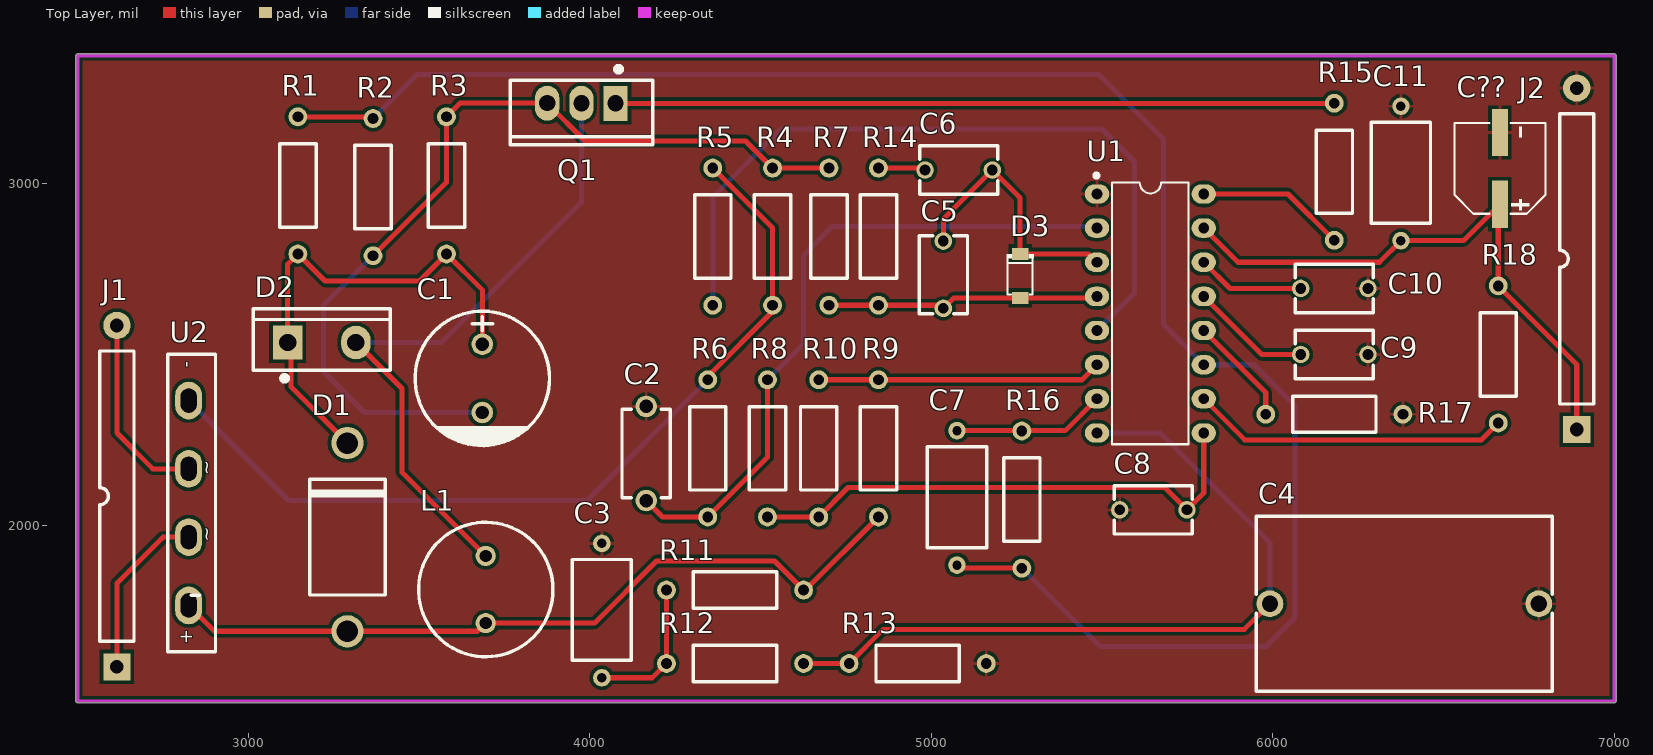
[diagram p0: Top Layer view]
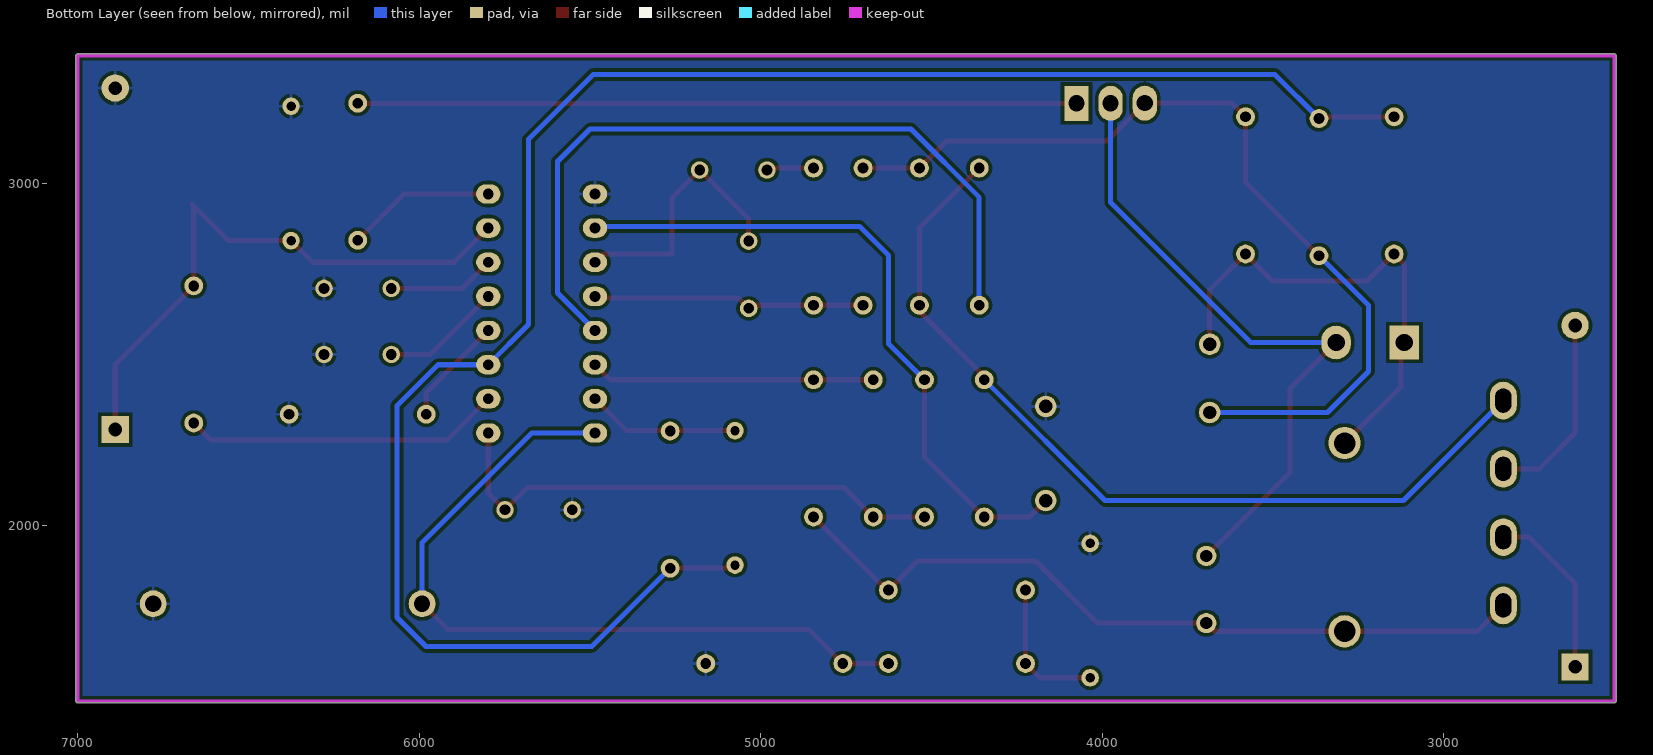
[diagram p1: Bottom Layer view, seen from below]
# Altium PCB MISC82375-2.PcbDoc
Units mil, origin at the board's own origin, x right, y up, seen from the top; angles counter-clockwise.
Board outline 4510.03 x 1900.03 mil, 2 copper layers (Top Layer, Bottom Layer); 39 components, 26 nets, 95 pads, 0 vias.

## Layer stack, top to bottom (the 12.6 mil dielectric is the usual default, probably not edited)
Top Solder: solder mask 0.4, Solder Resist, Dk 3.5
Top Layer: signal copper 1.4
Dielectric 1: dielectric 12.6, FR-4, Dk 4.8
Bottom Layer: signal copper 1.4
Bottom Solder: solder mask 0.4, Solder Resist, Dk 3.5

## Board outline
2494.99,1485 ccw(c2500,1485) 2500,1479.98 7000,1479.98 ccw(c7000,1485) 7005.02,1485 7005.02,3375 ccw(c7000,3375) 7000,3380.01 2500,3380.01 ccw(c2500,3375) 2494.99,3375

## Design rules (kind name [scope] priority, off if disabled: settings)
Clearance [All] p1: gap=10
MinimumSolderMaskSliver [All] p1: minsoldermaskwidth=0
PolygonConnect [All] p1: connectstyle=Relief reliefconductorwidth=10 reliefentries=4 polygonreliefangle="90 Angle" airgapwidth=10
RoutingVias [All] p1: holewidth=28 width=50 viastyle="Through Hole" minholewidth=28 minwidth=50 maxholewidth=28 maxwidth=50
SilkToSilkClearance [All] p1: silktosilkclearance=0
SilkToSolderMaskClearance [IsPad] p1: minsilkscreentomaskgap=0 clearancetoexposedcopper=TRUE
SolderMaskExpansion [All] p1: expansion=4
Width [All] p1: maxlimit=30 minlimit=10 preferedwidth=10
27 further rules are at their usual default settings.

## Components (designator, comment, footprint, x,y, rotation, side; value= is the part's Value field where it differs from the comment)
C1 "LKME1402A101MF" CAP-TH_BD10.0-P5.00-D1.0-FD 3685,2430 r270 top
C2 "KJKF222M2FF7035A075E" CAP-TH_L6.5-W3.5-P7.50-D1.0 4165,2210 r270 top
C3 "KY1102M400VAC70Y10093" CAP-TH_L7.5-W4.5-P10.00-D0.6 4035,1750 r270 top
C4 "CBB21-400V/255JP20" CAP-TH_L22.0-W12.5-P20.00-D0.7-FD 6385,1770 r180 top
C5 "178MU0002" CAP-TH_L5.8-W3.6-P5.0-D0.6 5035,2733.42 r90 top
C6 "178MU0002" CAP-TH_L5.8-W3.6-P5.0-D0.6 5080,3040 r180 top
C7 "KY1102M400VAC70Y10093" CAP-TH_L7.5-W4.5-P10.00-D0.6 5075,2080 r270 top
C8 "178MU0002" CAP-TH_L5.8-W3.6-P5.0-D0.6 5650,2045 r0 top
C9 "178MU0002" CAP-TH_L5.8-W3.6-P5.0-D0.6 6180,2500 r0 top
C10 "178MU0002" CAP-TH_L5.8-W3.6-P5.0-D0.6 6180,2693.43 r0 top
C11 "KY1102M400VAC70Y10093" CAP-TH_L7.5-W4.5-P10.00-D0.6 6375,3030 r270 top
C?? "RVE100UF35V67RV0072" CAP-SMD_BD6.3-L6.6-W6.6-LS7.6-FD-1 6665,3044.89 r90 top
D1 "1N5406_C5338388" DO-27_BD5.2-L8.9-P12.90-D1.5-RD 3290,1965 r270 top
D2 "GC3D10060A" TO-220-2_L10.2-W4.5-P5.08-L-A 3215,2535 r0 top
D3 "BZT52C8V2_C19077406" SOD-123_L2.7-W1.6-LS3.7-RD 5260,2730 r270 top
J1 "HOLE" DIP2 2615,1585 r90 top
J2 "HOLE" DIP2 6890,2280 r90 top
L1 "XR8*10-101K-L" IND-TH_BD10.0-P5.00-D0.6 3695,1811.57 r90 top
Q1 "IRF530NPBF" TO-220-3_L10.0-W4.5-P2.54-L 3975.01,3235.61 r180 top
R1 "MF1/4W-100K±1%-OT26" RES-TH_BD2.7-L6.2-P10.20-D0.4 3145,2995 r270 top
R2 "MF1/4W-100K±1%-OT26" RES-TH_BD2.7-L6.2-P10.20-D0.4 3365,2990 r90 top
R3 "MF1/4W-100K±1%-OT26" RES-TH_BD2.7-L6.2-P10.20-D0.4 3580,2995 r270 top
R4 "MF1/4W-100K±1%-OT26" RES-TH_BD2.7-L6.2-P10.20-D0.4 4535,2845 r90 top
R5 "MF1/4W-100K±1%-OT26" RES-TH_BD2.7-L6.2-P10.20-D0.4 4360,2845 r90 top
R6 "MF1/4W-100K±1%-OT26" RES-TH_BD2.7-L6.2-P10.20-D0.4 4345,2225 r90 top
R7 "MF1/4W-100K±1%-OT26" RES-TH_BD2.7-L6.2-P10.20-D0.4 4700,2845 r90 top
R8 "MF1/4W-100K±1%-OT26" RES-TH_BD2.7-L6.2-P10.20-D0.4 4520,2225 r90 top
R9 "MF1/4W-100K±1%-OT26" RES-TH_BD2.7-L6.2-P10.20-D0.4 4845,2225 r270 top
R10 "MF1/4W-100K±1%-OT26" RES-TH_BD2.7-L6.2-P10.20-D0.4 4670,2225 r270 top
R11 "MF1/4W-100K±1%-OT26" RES-TH_BD2.7-L6.2-P10.20-D0.4 4425,1810 r0 top
R12 "MF1/4W-100K±1%-OT26" RES-TH_BD2.7-L6.2-P10.20-D0.4 4425,1595 r0 top
R13 "MF1/4W-100K±1%-OT26" RES-TH_BD2.7-L6.2-P10.20-D0.4 4960,1595 r180 top
R14 "MF1/4W-100K±1%-OT26" RES-TH_BD2.7-L6.2-P10.20-D0.4 4845,2845 r90 top
R15 "MF1/4W-100K±1%-OT26" RES-TH_BD2.7-L6.2-P10.20-D0.4 6180,3035 r270 top
R16 "MF1/4W-100K±1%-OT26" RES-TH_BD2.7-L6.2-P10.20-D0.4 5265,2075 r270 top
R17 "MF1/4W-100K±1%-OT26" RES-TH_BD2.7-L6.2-P10.20-D0.4 6180,2325 r0 top
R18 "MF1/4W-100K±1%-OT26" RES-TH_BD2.7-L6.2-P10.20-D0.4 6660,2500 r90 top
U1 "UC3854N" PDIP-16_L19.3-W6.4-P2.54-LS7.94-BL 5641.3,2620 r270 top
U2 "GBU8K" GBU_4P-L22.0-W3.5-P5.08-GBU4K 2825,2065 r270 top

## Footprints (in the part's own frame and the unit in brackets; to place one, negate y for a bottom-side part, rotate by r counter-clockwise, add the part's x,y. Pads: shape width x height; smd on the part's side, far side on the other; paste and mask are expansions set on the pad)
CAP-SMD_BD6.3-L6.6-W6.6-LS7.6-FD-1 [mm]
  rect 3.5x1.2 smd: 1(-2.67,0) 2(2.67,0)
  silkscreen extent -3.38,-3.38 3.38,3.38
CAP-TH_BD10.0-P5.00-D1.0-FD [mm]
  round 1.6 hole 1: 1(-2.54,0) 2(2.54,0)
  silkscreen extent -5,-5 5.08,5
CAP-TH_L5.8-W3.6-P5.0-D0.6 [mm]
  round 1.3 hole 0.8 paste+0 mask+0.05: 1(-2.5,0)
  round 1.3 hole 0.8 copper offset 0,0 paste+0 mask+0.05: 2(2.5,0)
  silkscreen extent -2.9,-1.8 2.9,1.8
CAP-TH_L6.5-W3.5-P7.50-D1.0 [mm]
  round 1.6 hole 1: 1(-3.5,0) 2(3.5,0)
  silkscreen extent -3.3,-1.8 3.3,1.8
CAP-TH_L7.5-W4.5-P10.00-D0.6 [mm]
  round 1.3 hole 0.7: 1(-5,0) 2(5,0)
  silkscreen extent -3.8,-2.2 3.7,2.2
CAP-TH_L22.0-W12.5-P20.00-D0.7-FD [mm]
  round 2 hole 1.2: 1(-10,0) 2(10,0)
  silkscreen extent -11,-6.5 11,6.5
DIP2 [mil]
  rect 80x80 hole 40: 1(0,0)
  round 80 hole 40: 2(1000,0)
  silkscreen extent 75,-50 925,50
DO-27_BD5.2-L8.9-P12.90-D1.5-RD [mm]
  round 2.4 hole 1.6: 1(-7,0) 2(7,0)
  silkscreen extent -4.3,-2.8 4.3,2.8
GBU_4P-L22.0-W3.5-P5.08-GBU4K [mm]
  oval 2.8x2 hole 1.2 slot 1.8 at 0 deg: 1(-7.62,0) 2(-2.54,0) 3(2.54,0) 4(7.62,0)
  silkscreen extent -11.05,-1.56 11.05,2
IND-TH_BD10.0-P5.00-D0.6 [mm]
  round 1.5 hole 0.9 paste+0 mask+0.05: 1(-2.5,0) 2(2.5,0)
  silkscreen extent -5,-5 5,5
PDIP-16_L19.3-W6.4-P2.54-LS7.94-BL [mm]
  oval 1.44x1.8 hole 0.8: 1(-8.89,-3.97) 2(-6.35,-3.97) 3(-3.81,-3.97) 4(-1.27,-3.97) 5(1.27,-3.97) 6(3.81,-3.97) 7(6.35,-3.97) 8(8.89,-3.97) 9(8.89,3.97) 10(6.35,3.97) 11(3.81,3.97) 12(1.27,3.97) 13(-1.27,3.97) 14(-3.81,3.97) 15(-6.35,3.97) 16(-8.89,3.97)
  silkscreen extent -10.41,-4.17 9.73,2.84
RES-TH_BD2.7-L6.2-P10.20-D0.4 [mm]
  round 1.4 hole 0.8 copper offset 0,0: 1(-5.1,0) 2(5.1,0)
  silkscreen extent -3.1,-1.35 3.1,1.35
SOD-123_L2.7-W1.6-LS3.7-RD [mm]
  rect 0.91x1.22 smd: 1(-1.635,0) 2(1.635,0)
  silkscreen extent -1.6,-1 1.38,1
TO-220-2_L10.2-W4.5-P5.08-L-A [mm]
  rect 2.2x2.5 hole 1.3: 1(-2.54,0)
  oval 2.2x2.5 hole 1.3: 3(2.54,0)
  silkscreen extent -5.1,-2.86 5.1,2.5
TO-220-3_L10.0-W4.5-P2.54-L [mm]
  rect 1.8x2.6 hole 1.2: 1(-2.54,0.005)
  oval 1.8x2.6 hole 1.2: 2(0,0.005)
  oval 1.8x2.6 hole 1.2 copper offset 0,0: 3(2.54,-0.005)
  silkscreen extent -5.3,-2.73 5.3,3.09

## Part data
J1 J2: library part J

## Nets (pads, with @x,y where several pads share a name; then routed paths per layer and width w, separated by ;. In a path a pad name is that pad's centre, name@x,y a point inside that pad or via, vN(x,y) a via of type N, cw(c..) or ccw(c..) an arc to the next point about the centre after c; other vN are vias at no path point)
GND: C2.1 C3.1 C4.1 C8.1 C9.2 C10.2 C11.1 C??.2 J2.2 R13.1 R17.2 U1.1
NetC1_1: C1.1 D1.1 D2.1 R1.2 R3.2 | length 1446.8
  Top Layer w15: D1.1 3125,2405.58 3125,2525 D2.1 3115,2764.2 R1.2 3224.2,2715 3500.8,2715 R3.2 3685,2689.2 C1.1
NetC1_2: C1.2 Q1.3 R2.1 R3.1 R4.2 R7.2 | length 2624.9
  Top Layer w15: R2.1 3580,3004.2 R3.1 3620,3235.8 Q1.3 3985.8,3125 4455.8,3125 R4.2 R7.2
  Bottom Layer w15: R2.1 3220,2644.2 3220,2450 3340,2330 C1.2
NetC2_2: C2.2 R6.1 R8.2 U1.2 | length 1978.9
  Top Layer w15: C2.2 4213,2024.2 R6.1 4520,2199.2 R8.2
  Bottom Layer w15: R8.2 4625,2530.8 4625,2790 4709.93,2874.93 5480.07,2874.93 U1.2
NetC3_2: C3.2 R11.1 R12.1 | length 421.5
  Top Layer w15: C3.2 4182.35,1553.15 R12.1 R11.1
NetC4_2: C4.2 R12.2 R13.2 U1.8 | length 2256.1
  Top Layer w15: R12.2 R13.2 4859.2,1695 5916.31,1695 C4.2
  Bottom Layer w15: U1.8 5670,2270 5991.3,1948.7 C4.2
NetC5_1: C5.1 D3.2 R7.1 R14.1 U1.4 | length 803.3
  Top Layer w15: R7.1 R14.1 5025.8,2644.2 C5.1 5065.63,2665.63 D3.2 5480.63,2665.63 U1.4
NetC5_2: C5.2 C6.1 D3.1 U1.3 | length 782.1
  Top Layer w15: C5.2 5035,2896.58 C6.1 5260,2958.42 D3.1 5460.62,2794.37 U1.3
NetC6_2: C6.2 R14.2 | length 139
  Top Layer w15: R14.2 4975.77,3045.8 C6.2
NetC7_1: C7.1 R16.1 U1.7 | length 448.6
  Top Layer w15: C7.1 5391.85,2276.85 U1.7
NetC7_2: C7.2 R1.1 R2.2 R16.2 U1.11 | length 5439
  Top Layer w15: R1.1 3360,3195.8 R2.2 ; C7.2 5083.95,1874.2 R16.2
  Bottom Layer w15: R2.2 3494.2,3320 5490,3320 5680,3130 5680,2587.6 U1.11 5945,2470 6065,2350 6065,1730 5980,1645 5494.2,1645 R16.2
NetC8_2: C8.2 R8.1 R10.2 U1.9 | length 1536.3
  Top Layer w15: R8.1 R10.2 4755.8,2110 5683.43,2110 C8.2 5797.6,2094.17 U1.9
NetC9_1: C9.1 U1.13 | length 354.4
  Top Layer w15: U1.13 5967.6,2500 C9.1
NetC10_1: C10.1 U1.14 | length 315.7
  Top Layer w15: U1.14 5874.17,2693.43 C10.1
NetC11_2: C11.2 C??.1 J2.1 R18.2 U1.15 | length 1729.2
  Top Layer w15: U1.15 5897.6,2770 6311.85,2770 C11.2 6558.38,2833.15 C??.1@6660,2934.77 ; C??.1 C??.1@6660,2934.77 ; J2.1 6890,2470.8 R18.2 C??.1@6660,2934.77
NetD1_2: D1.2 L1.1 R9.2 R11.2 U2.4 | length 2260.4
  Top Layer w15: U2.4 2900.58,1689.42 D1.2 3671.27,1689.42 L1.1 4013.15,1713.15 4195,1895 4540.8,1895 R11.2 4630.8,1810 R9.2
NetD2_3: D2.3 L1.2 Q1.2 | length 1902.7
  Top Layer w15: D2.3 3450,2400 3450,2155 L1.2
  Bottom Layer w15: D2.3 3565,2535 3975.02,2945.02 Q1.2
NetJ1_4: J1.1 U2.3 | length 510.9
  Top Layer w15: J1.1 2615,1830 2750,1965 U2.3
NetJ1_5: J1.2 U2.2 | length 568.5
  Top Layer w15: J1.2 2615,2270 2720,2165 U2.2
NetQ1_1: Q1.1 R15.1 | length 2105.1
  Top Layer w15: Q1.1 6179.61,3235.41 R15.1
NetR4_1: R4.1 R5.2 R6.2 U2.1 | length 2548.9
  Top Layer w15: R6.2@4345,2435.8 4535,2625.8 R4.1 4535,2870.8 R5.2
  Bottom Layer w15: U2.1 3117.8,2072.2 3991.39,2072.2 R6.2
NetR5_1: R5.1 U1.5 | length 2213.6
  Bottom Layer w15: R5.1 4360,2960 4560,3160 5500,3160 5595,3065 5595,2680 U1.5
NetR9_1: R9.1 R10.1 U1.6 | length 833.3
  Top Layer w15: R10.1 R9.1 5440.8,2425.8 U1.6
NetR15_2: R15.2 U1.16 | length 438.6
  Top Layer w15: U1.16 6044.2,2970 R15.2
NetR17_1: R17.1 U1.12 | length 320.2
  Top Layer w15: U1.12 5979.2,2388.4 R17.1
NetR18_1: R18.1 U1.10 | length 932.5
  Top Layer w15: U1.10 5917.6,2250 6610.8,2250 R18.1

## Polygon pours and split planes (outlines as drawn)
GND on Bottom Layer "G" (solid, remove dead copper, pour order 0): 1705,3875 1920,3660 7320,3660 7320,1415 7135,1230 7035,1330 1965,1330
GND on Top Layer "G" (solid, remove dead copper, pour order 2): 2160,3700 7275,3700 7380,3595 7040,3255 7040,975 2270,975 2200,1045

## Keep-outs
Keep-Out Layer:
  lines w10: 2500,3275 2500,3375 7000,3375 7000,1485 2500,1485 2500,3295